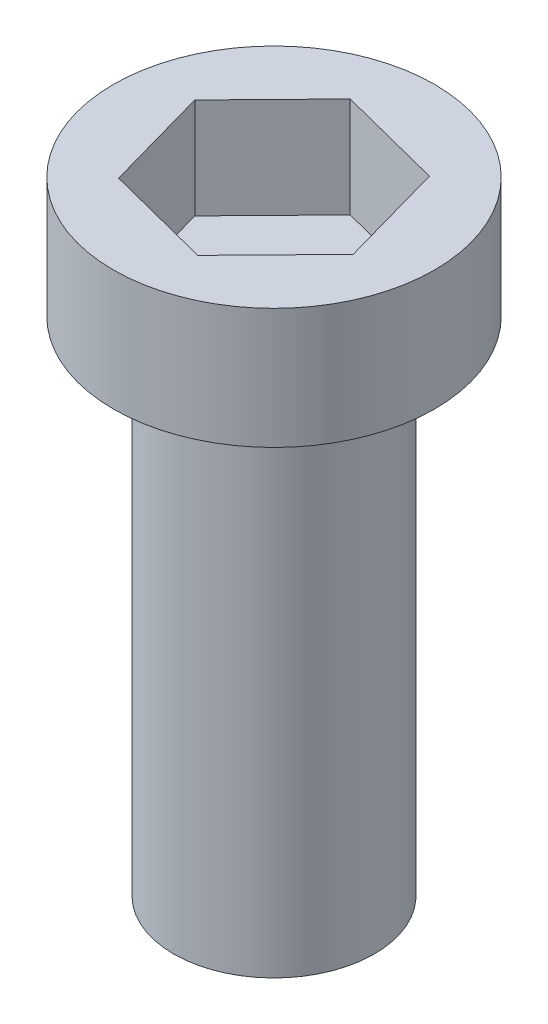
from build123d import *

# Parameters (mm, degrees)
SKETCH1_R           = 5
BOSS_EXTRUDE1_DEPTH = 25
SKETCH2_R           = 8
BOSS_EXTRUDE2_DEPTH = 6
CUT_EXTRUDE1_DEPTH  = 5


with BuildPart() as part:
    # Sketch1 → Boss-Extrude1 (new body)
    with BuildSketch(Plane(origin=(0, 0, 0), x_dir=(1, 0, 0), z_dir=(0, 1, 0))):
        with Locations(Location((0, 0, 0), (0, 0, 270))):
            Circle(SKETCH1_R)
    extrude(amount=BOSS_EXTRUDE1_DEPTH)

    # Sketch2 → Boss-Extrude2 (add)
    with BuildSketch(Plane(origin=(0, 25, 0), x_dir=(1, 0, 0), z_dir=(0, 1, 0))):
        with Locations(Location((0, 0, 0), (0, 0, 270))):
            Circle(SKETCH2_R)
    extrude(amount=BOSS_EXTRUDE2_DEPTH)

    # Sketch3 → Cut-Extrude1 (cut)
    with BuildSketch(Plane(origin=(0, 31, 0), x_dir=(1, 0, 0), z_dir=(0, 1, 0))):
        Polygon((-1.474961989, 5.269810816), (-5.301271034, 1.357550856), (-3.826309045, -3.91225996), (1.474961989, -5.269810816), (5.301271034, -1.357550856), (3.826309045, 3.91225996), align=None)
    extrude(amount=-CUT_EXTRUDE1_DEPTH, mode=Mode.SUBTRACT)


solid = part.part
